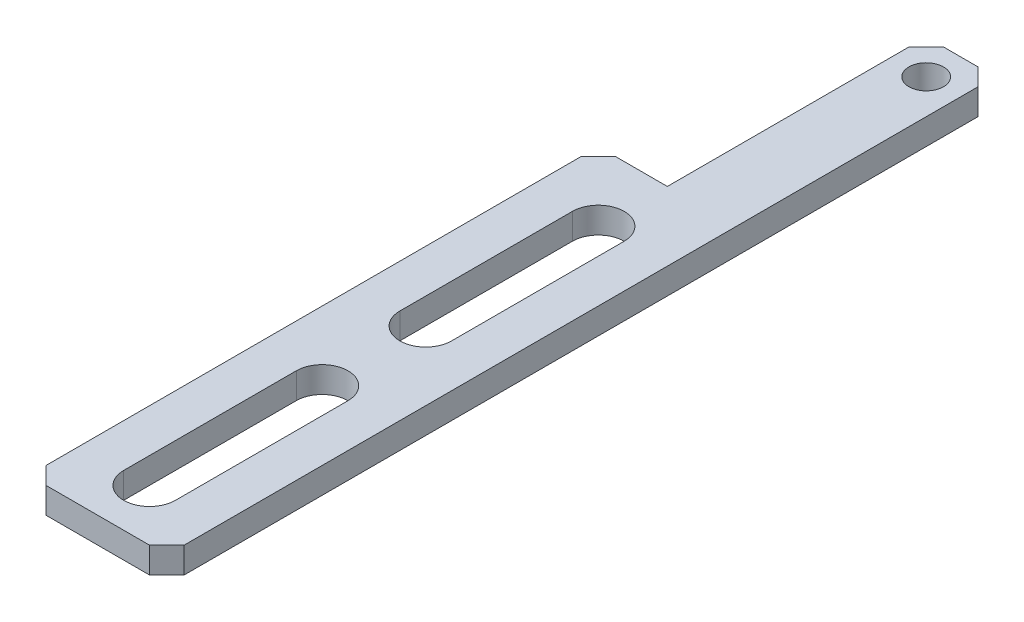
SolidWorks part; units mm, degrees
ref_plane "Front Plane" through (0, 0, 0) normal (0, 0, 1) x (1, 0, 0)
ref_plane "Top Plane" through (0, 0, 0) normal (0, 1, 0) x (1, 0, 0)
ref_plane "Right Plane" through (0, 0, 0) normal (1, 0, 0) x (0, 0, -1)
sketch "Sketch1" plane through (0, 0, 0) normal (0, 1, 0) x (1, 0, 0)
  line L1 (0, 0) -> (8, 0)
  line L2 (0, 0) -> (0, 48)
  line L3 (0, 48) -> (8, 48)
  line L4 (8, 0) -> (8, 48)
  dimension "D1" = 8
  dimension "D2" = 48
extrude "Boss-Extrude1" add sketch "Sketch1" along normal blind 1.5
hole_wizard "Ø2.5 (2.5) Diameter Hole1" positions "Sketch4" profile "Sketch5" hole size "Ø2.5" standard "Gb"
sketch "Sketch4" plane through (0, 1.5, 0) normal (0, 1, 0) x (1, 0, 0)
  line L0 (8, 48) -> (0, 48) construction
  line L1 (8, 0) -> (8, 48) construction
  point P0 (6, 46)
  dimension "D1" = 2
  dimension "D2" = 2
sketch "Sketch5" plane through (6, 1.5, -46) normal (1, 0, 0) x (0, 0, 1)
  line L0 (0, 0) -> (0, 5.6009)
  line L1 (0, 5.6009) -> (1, 5)
  line L2 (1, 5) -> (1, 0)
  line L5 (1, 0) -> (0, 0)
  line L10 (0, 5.6009) -> (-1, 5) construction
  line L11 (0, -6.35) -> (0, 107.95) construction
  dimension "孔直径" = 2
  dimension "孔深度" = 5
  dimension "导头角度" = 118
sketch "Sketch6" plane through (0, 1.5, 0) normal (0, 1, 0) x (1, 0, 0)
  line L0 (0, 48) -> (0, 0) construction
  line L1 (0, 48) -> (4, 48)
  line L2 (0, 48) -> (0, 33)
  line L3 (0, 33) -> (4, 33)
  line L4 (4, 48) -> (4, 33)
  line L5 (8, 48) -> (0, 48) construction
  dimension "D1" = 15
  dimension "D2" = 4
extrude "Cut-Extrude1" cut sketch "Sketch6" against normal blind 10
sketch "Sketch7" plane through (0, 1.5, 0) normal (0, 1, 0) x (1, 0, 0)
  line L0 (0, 0) -> (8, 0) construction
  line L1 (0, 33) -> (0, 0) construction
  circle A0 centre (4, 24) radius 1.5
  circle A1 centre (4, 8) radius 1.5
  dimension "D4" = 3
  dimension "D1" = 16
  dimension "D2" = 8
  dimension "D3" = 4
extrude "Cut-Extrude2" cut sketch "Sketch7" against normal blind 10
chamfer "Chamfer1" distance 1 angle 45 5 edges at (8, 0.75, -48) (8, 0.75, 0) (0, 0.75, 0) (0, 0.75, -33) (4, 0.75, -48)
sketch "Sketch8" plane through (0, 1.5, 0) normal (0, 1, 0) x (1, 0, 0)
  line L0 (4, 29) -> (4, 19) construction
  line L1 (5.5, 29) -> (5.5, 19)
  line L2 (2.5, 29) -> (2.5, 19)
  line L3 (4, 3) -> (4, 13) construction
  line L4 (2.5, 3) -> (2.5, 13)
  line L5 (5.5, 3) -> (5.5, 13)
  arc A0 (5.5, 29) -> (2.5, 29) centre (4, 29) ccw
  arc A1 (2.5, 19) -> (5.5, 19) centre (4, 19) ccw
  arc A2 (2.5, 3) -> (5.5, 3) centre (4, 3) ccw
  arc A3 (5.5, 13) -> (2.5, 13) centre (4, 13) ccw
  point P2 (4, 24)
  point P9 (4, 8)
  dimension "D1" = 10
  dimension "D2" = 3
extrude "Cut-Extrude3" cut sketch "Sketch8" against normal blind 10
